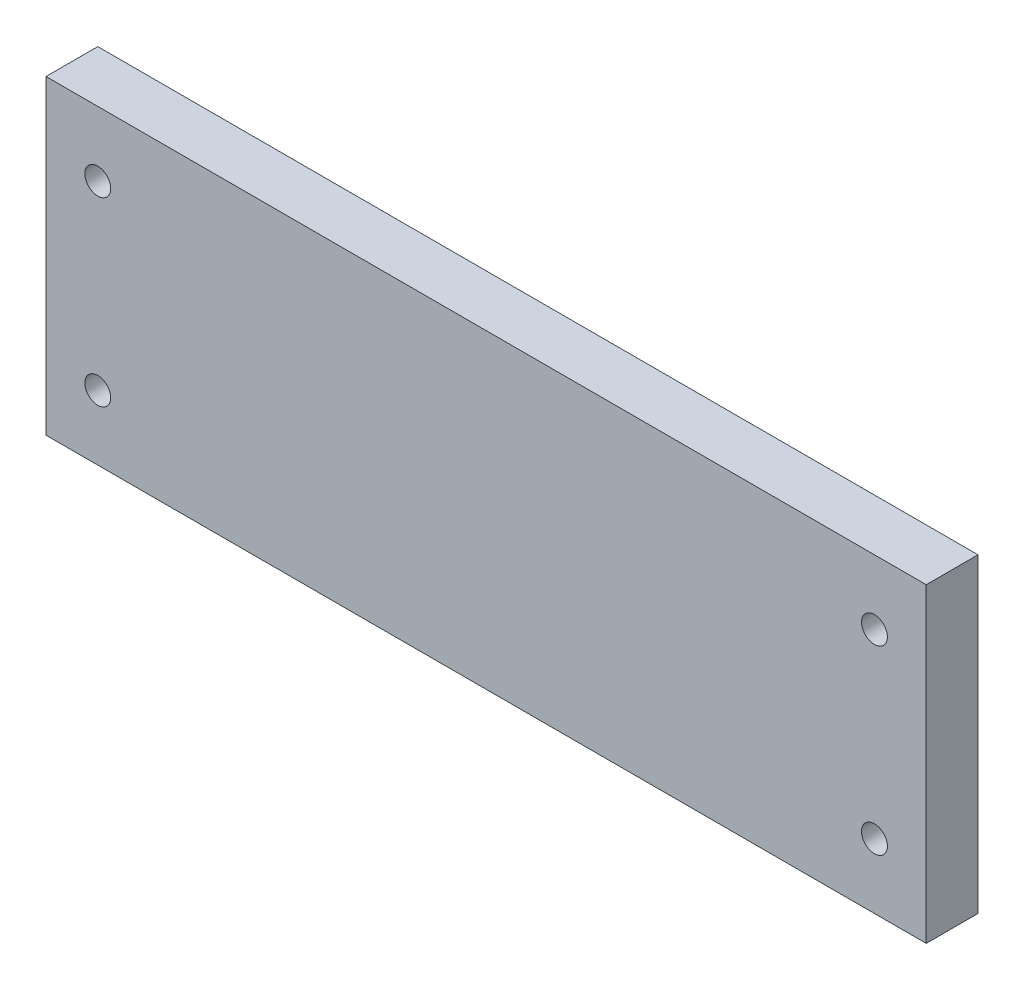
from build123d import *

# Parameters (mm, degrees)
SKETCH1_W           = 340
SKETCH1_H           = 120
SKETCH1_R           = 5
BOSS_EXTRUDE1_DEPTH = 20


with BuildPart() as part:
    # Sketch1 → Boss-Extrude1 (new body)
    with BuildSketch(Plane.XY):
        with Locations((170, 60)):
            Rectangle(SKETCH1_W, SKETCH1_H)
        with Locations((20, 95)):
            Circle(SKETCH1_R, mode=Mode.SUBTRACT)
        with Locations((320, 95)):
            Circle(SKETCH1_R, mode=Mode.SUBTRACT)
        with Locations((320, 25)):
            Circle(SKETCH1_R, mode=Mode.SUBTRACT)
        with Locations((20, 25)):
            Circle(SKETCH1_R, mode=Mode.SUBTRACT)
    extrude(amount=BOSS_EXTRUDE1_DEPTH)


solid = part.part
